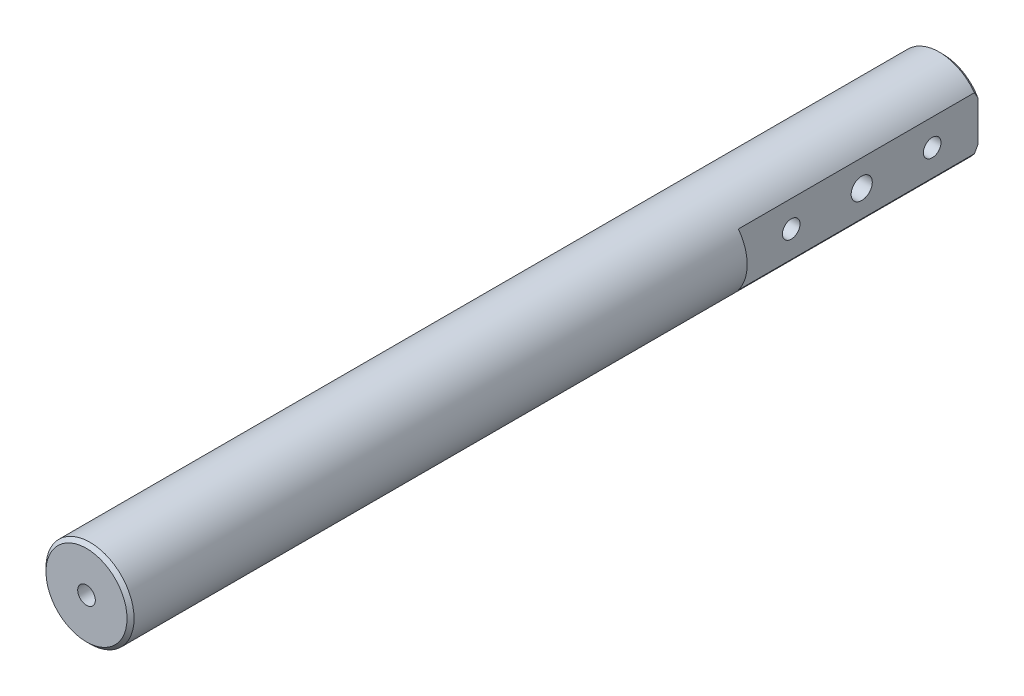
from build123d import *

# Parameters (mm, degrees)
SKETCH1_R             = 12.5
BOSS_EXTRUDE1_DEPTH   = 243
SKETCH2_W             = 20
SKETCH2_H             = 15
CUT_EXTRUDE1_DEPTH    = 68
M6_TAPPED_HOLE1_D     = 5
M6_TAPPED_HOLE1_DEPTH = 15
M6_TAPPED_HOLE1_TIP   = 1.502151548
M6_TAPPED_HOLE2_D     = 5
M6_TAPPED_HOLE2_DEPTH = 15
M6_TAPPED_HOLE2_TIP   = 1.502151548
SKETCH7_W             = 2.5
SKETCH7_H             = 15
CUT_EXTRUDE2_DEPTH    = 160
M4_TAPPED_HOLE1_D     = 3.3
M4_TAPPED_HOLE1_DEPTH = 10.1
M4_TAPPED_HOLE1_TIP   = 0.991420021
SKETCH10_R            = 3
CUT_EXTRUDE3_DEPTH    = 10
CHAMFER1_SIZE         = 1


with BuildPart() as part:
    # Sketch1 → Boss-Extrude1 (new body)
    with BuildSketch(Plane.XY):
        Circle(SKETCH1_R)
    extrude(amount=BOSS_EXTRUDE1_DEPTH)

    # Sketch2 → Cut-Extrude1 (cut)
    with BuildSketch(Plane.XY):
        with Locations((20, 0)):
            Rectangle(SKETCH2_W, SKETCH2_H)
    extrude(amount=CUT_EXTRUDE1_DEPTH, mode=Mode.SUBTRACT)

    # M6 Tapped Hole1
    with Locations(Plane.XY.offset(243)):
        with Locations((0, 0)):
            Hole(M6_TAPPED_HOLE1_D / 2, depth=M6_TAPPED_HOLE1_DEPTH)
            with Locations((0, 0, -(M6_TAPPED_HOLE1_DEPTH + M6_TAPPED_HOLE1_TIP / 2))):  # 118° drill point
                Cone(0, M6_TAPPED_HOLE1_D / 2, M6_TAPPED_HOLE1_TIP, mode=Mode.SUBTRACT)

    # M6 Tapped Hole2
    with Locations(Plane(origin=(10, 0, 0), x_dir=(0, 0, -1), z_dir=(1, 0, 0))):
        with Locations((-13, 0), (-53, 0)):
            Hole(M6_TAPPED_HOLE2_D / 2, depth=M6_TAPPED_HOLE2_DEPTH)
            with Locations((0, 0, -(M6_TAPPED_HOLE2_DEPTH + M6_TAPPED_HOLE2_TIP / 2))):  # 118° drill point
                Cone(0, M6_TAPPED_HOLE2_D / 2, M6_TAPPED_HOLE2_TIP, mode=Mode.SUBTRACT)

    # Sketch7 → Cut-Extrude2 (cut)
    with BuildSketch(Plane(origin=(0, 0, 0), x_dir=(-1, 0, 0), z_dir=(0, 0, -1))):
        with Locations((11.25, 0)):
            Rectangle(SKETCH7_W, SKETCH7_H)
    extrude(amount=-CUT_EXTRUDE2_DEPTH, mode=Mode.SUBTRACT)

    # M4 Tapped Hole1
    with Locations(Plane.ZY.offset(10)):
        with Locations((8, 0), (83, 0), (48, 0)):
            Hole(M4_TAPPED_HOLE1_D / 2, depth=M4_TAPPED_HOLE1_DEPTH)
            with Locations((0, 0, -(M4_TAPPED_HOLE1_DEPTH + M4_TAPPED_HOLE1_TIP / 2))):  # 118° drill point
                Cone(0, M4_TAPPED_HOLE1_D / 2, M4_TAPPED_HOLE1_TIP, mode=Mode.SUBTRACT)

    # Sketch10 → Cut-Extrude3 (cut)
    with BuildSketch(Plane(origin=(10, 0, 0), x_dir=(0, 0, -1), z_dir=(1, 0, 0))):
        with Locations((-33, 0)):
            Circle(SKETCH10_R)
    extrude(amount=-CUT_EXTRUDE3_DEPTH, mode=Mode.SUBTRACT)

    # Chamfer1
    chamfer1_edges = [part.edges().sort_by_distance(p)[0] for p in [
        (0, 12.5, 0),
        (0, -12.5, 0),
        (-12.5, 0, 243),
    ]]
    chamfer(chamfer1_edges, length=CHAMFER1_SIZE)


solid = part.part
